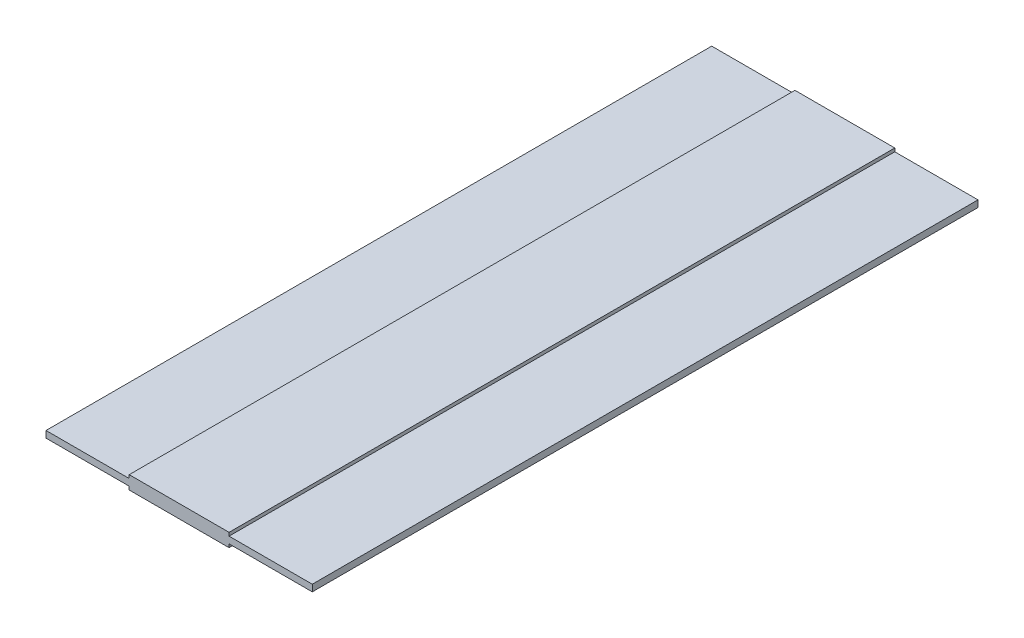
from build123d import *

# Parameters (mm, degrees)
SKETCH1_W           = 200
SKETCH1_H           = 5
BOSS_EXTRUDE1_DEPTH = 500
SKETCH2_W           = 75
SKETCH2_H           = 10
BOSS_EXTRUDE2_DEPTH = 500


with BuildPart() as part:
    # Sketch1 → Boss-Extrude1 (new body)
    with BuildSketch(Plane.XY):
        Rectangle(SKETCH1_W, SKETCH1_H)
    extrude(amount=BOSS_EXTRUDE1_DEPTH)

    # Sketch2 → Boss-Extrude2 (add)
    with BuildSketch(Plane.XY.offset(500)):
        Rectangle(SKETCH2_W, SKETCH2_H)
    extrude(amount=-BOSS_EXTRUDE2_DEPTH)


solid = part.part
